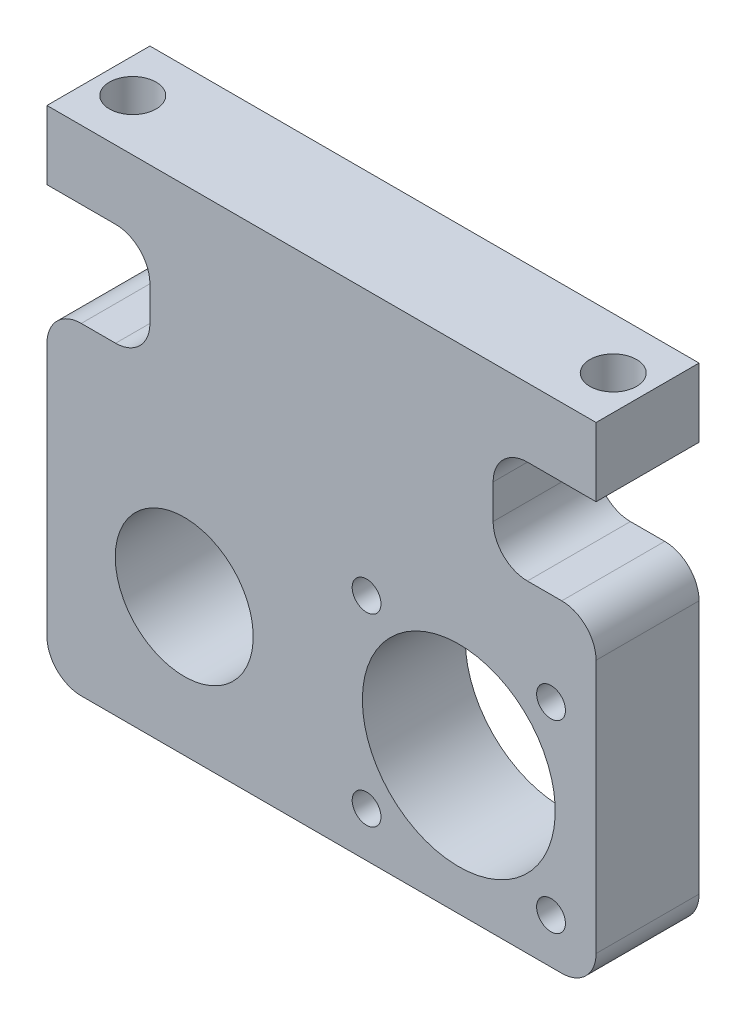
from build123d import *

# Parameters (mm, degrees)
BOSS_EXTRUDE1_DEPTH   = 7.5
CUT_EXTRUDE1_REACH    = 84.706
SKETCH2_R             = 3.4
SKETCH3_R             = 14.05
SKETCH3_R_2           = 10.05
CUT_EXTRUDE2_DEPTH    = 15
FILLET1_R             = 5
M5_TAPPED_HOLE1_D     = 4.2
BODY_MOVE_COPY1_ANGLE = 180


with BuildPart() as part:
    # Sketch1 → Boss-Extrude1 (new, symmetric)
    with BuildSketch(Plane.XY):
        Polygon((40, 0), (-40, 0), (-40, 10), (-25, 10), (-25, 25), (-40, 25), (-40, 72), (40, 72), (40, 25), (25, 25), (25, 10), (40, 10), align=None)
    extrude(amount=BOSS_EXTRUDE1_DEPTH, both=True)

    # Sketch2 → Cut-Extrude1 (cut, up to next)
    with BuildSketch(Plane.XZ, mode=Mode.PRIVATE) as cut_extrude1_sk1:
        with Locations(Location((-35, 0, 0), (0, 0, 270))):
            Circle(SKETCH2_R)
    cut_extrude1_tool1 = extrude(cut_extrude1_sk1.sketch, amount=-CUT_EXTRUDE1_REACH, mode=Mode.PRIVATE) & part.part
    # Sketch2 → Cut-Extrude1 (cut, up to next)
    with BuildSketch(Plane.XZ, mode=Mode.PRIVATE) as cut_extrude1_sk2:
        with Locations(Location((35, 0, 0), (0, 0, 270))):
            Circle(SKETCH2_R)
    cut_extrude1_tool2 = extrude(cut_extrude1_sk2.sketch, amount=-CUT_EXTRUDE1_REACH, mode=Mode.PRIVATE) & part.part
    add(cut_extrude1_tool1.solids().sort_by_distance((-35, 0, 0))[0], mode=Mode.SUBTRACT)
    add(cut_extrude1_tool2.solids().sort_by_distance((35, 0, 0))[0], mode=Mode.SUBTRACT)

    # Sketch3 → Cut-Extrude2 (cut)
    with BuildSketch(Plane.XY.offset(7.5)):
        with Locations((-20, 52)):
            Circle(SKETCH3_R)
        with Locations((20, 52)):
            Circle(SKETCH3_R_2)
    extrude(amount=-CUT_EXTRUDE2_DEPTH, mode=Mode.SUBTRACT)

    # Fillet1
    fillet1_edges = [part.edges().sort_by_distance(p)[0] for p in [
        (-25, 10, 0),
        (-25, 25, 0),
        (-40, 25, 0),
        (-40, 72, 0),
        (40, 72, 0),
        (40, 25, 0),
        (25, 25, 0),
        (25, 10, 0),
    ]]
    fillet(fillet1_edges, radius=FILLET1_R)

    # M5 Tapped Hole1 (through all)
    with Locations(Plane(origin=(0, 0, -7.5), x_dir=(-1, 0, 0), z_dir=(0, 0, -1))):
        with Locations((33.435028843, 38.564971157), (6.564971157, 38.564971157), (6.564971157, 65.435028843), (33.435028843, 65.435028843)):
            Hole(M5_TAPPED_HOLE1_D / 2)


with BuildPart() as part_1:
    # Body-Move/Copy1: moved
    add(part.part.rotate(Axis((0, 30, 0), (0, 0, 1)), BODY_MOVE_COPY1_ANGLE))


solid = part_1.part
